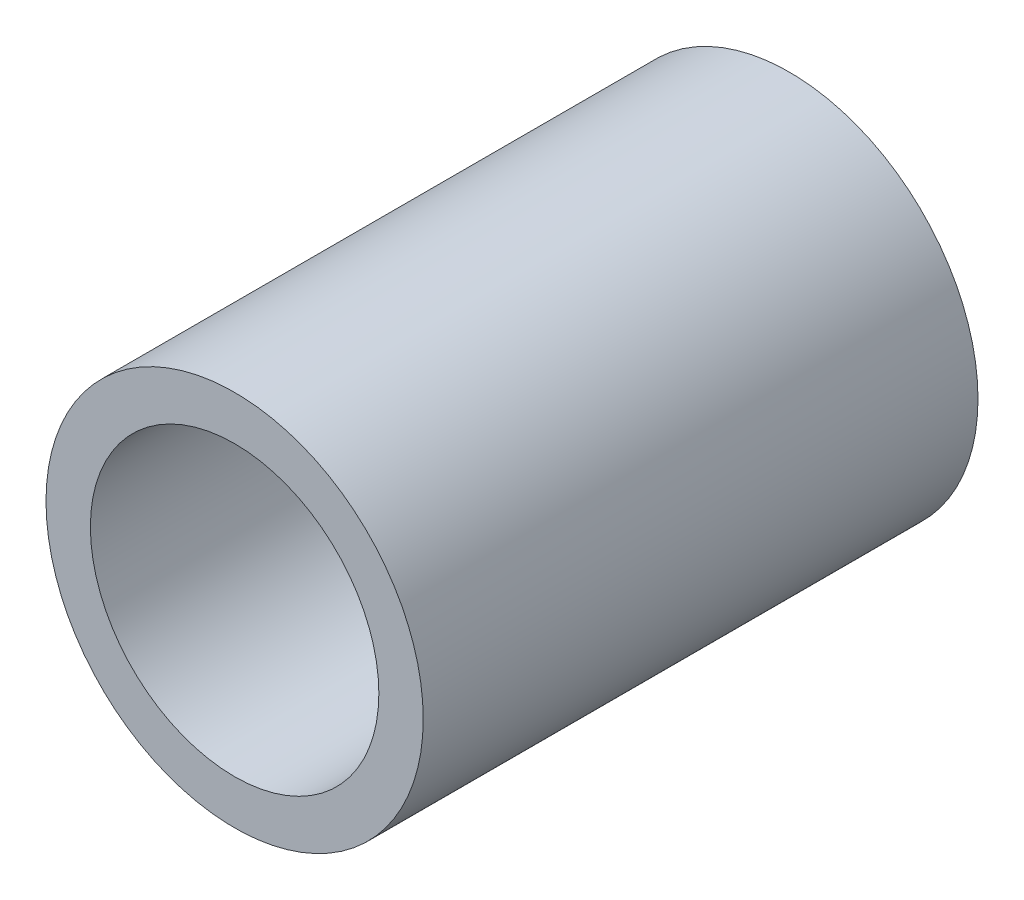
SolidWorks part; units mm, degrees
ref_plane "Front Plane" through (0, 0, 0) normal (0, 0, 1) x (1, 0, 0)
ref_plane "Top Plane" through (0, 0, 0) normal (0, 1, 0) x (1, 0, 0)
ref_plane "Right Plane" through (0, 0, 0) normal (1, 0, 0) x (0, 0, -1)
sketch "Sketch1" plane through (0, 0, 0) normal (0, 0, 1) x (1, 0, 0)
  circle A0 centre (0, 0) radius 17
  circle A1 centre (0, 0) radius 13
extrude "Boss-Extrude1" add sketch "Sketch1" along normal blind 50
